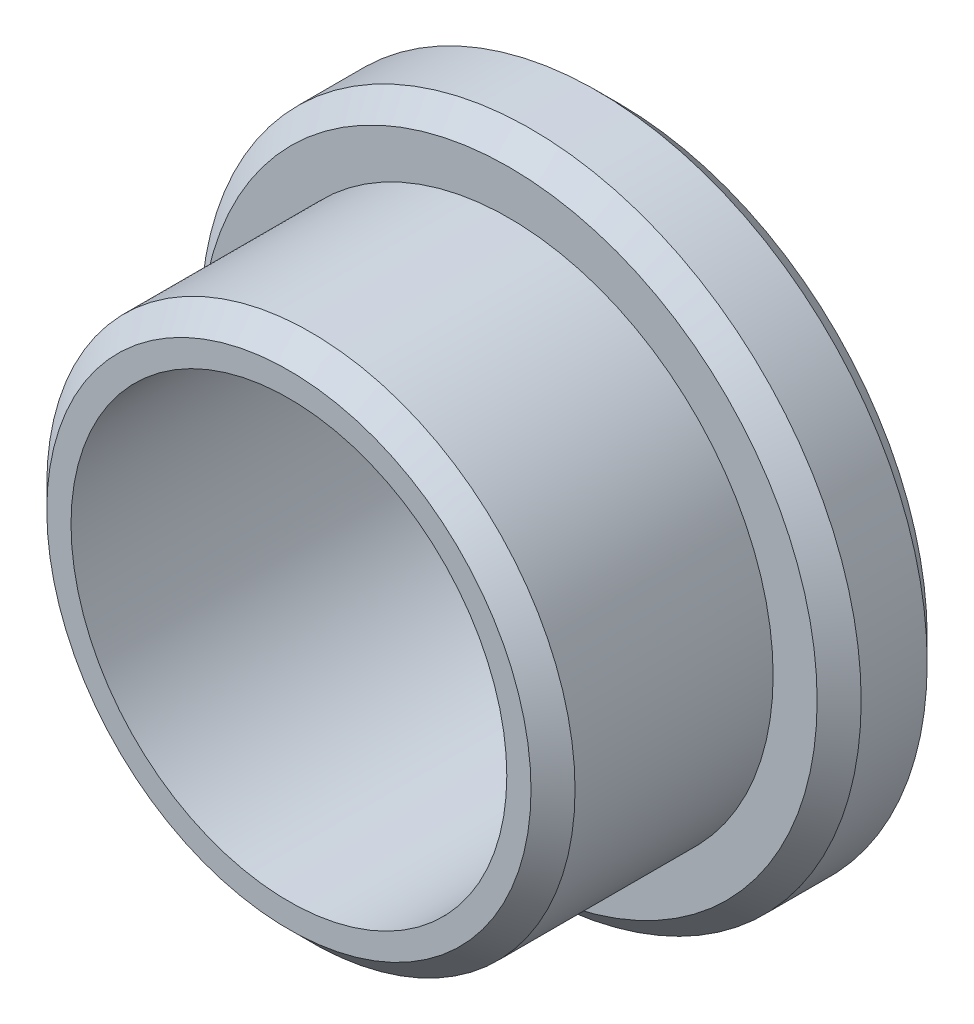
SolidWorks part; units mm, degrees
material "Plain carbon steel"
ref_plane "Front Plane" through (0, 0, 0) normal (0, 0, 1) x (1, 0, 0)
ref_plane "Top Plane" through (0, 0, 0) normal (0, 1, 0) x (1, 0, 0)
ref_plane "Right Plane" through (0, 0, 0) normal (1, 0, 0) x (0, 0, -1)
sketch "Sketch2" plane through (0, 0, 0) normal (0, 0, 1) x (1, 0, 0)
  circle A0 centre (0, 0) radius 15
  circle A1 centre (0, 0) radius 9.9
extrude "Boss-Extrude1" add sketch "Sketch2" along normal blind 5
sketch "Sketch3" plane through (0, 0, 5) normal (0, 0, 1) x (1, 0, 0)
  circle A0 centre (0, 0) radius 12
  circle A1 centre (0, 0) radius 9.9
extrude "Boss-Extrude2" add sketch "Sketch3" along normal blind 10
chamfer "Chamfer1" distance 1 distance2 1 3 edges at (12, 0, 15) (15, 0, 0) (15, 0, 5)
